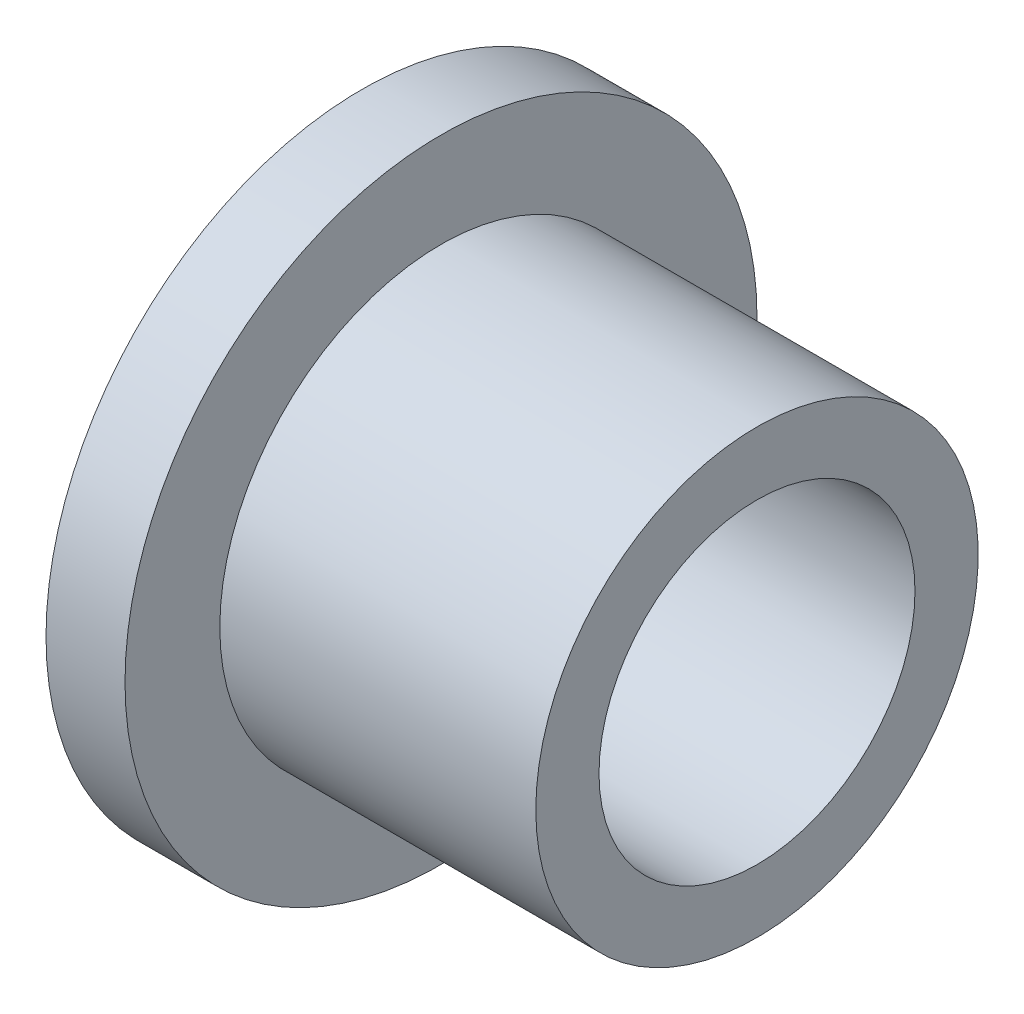
from build123d import *


with BuildPart() as part:
    # Sketch1 → Revolve1 (revolve)
    with BuildSketch(Plane(origin=(0, 0, 0), x_dir=(1, 0, 0), z_dir=(0, 1, 0)), mode=Mode.PRIVATE) as revolve1_sk:
        Polygon((0, 0), (0, 10), (5, 10), (5, 4), (25, 4), (25, 0), align=None)
    revolve(revolve1_sk.sketch.rotate(Axis((0, 0, 10), (1, 0, 0)), 180), axis=Axis((0, 0, 10), (1, 0, 0)))


solid = part.part
